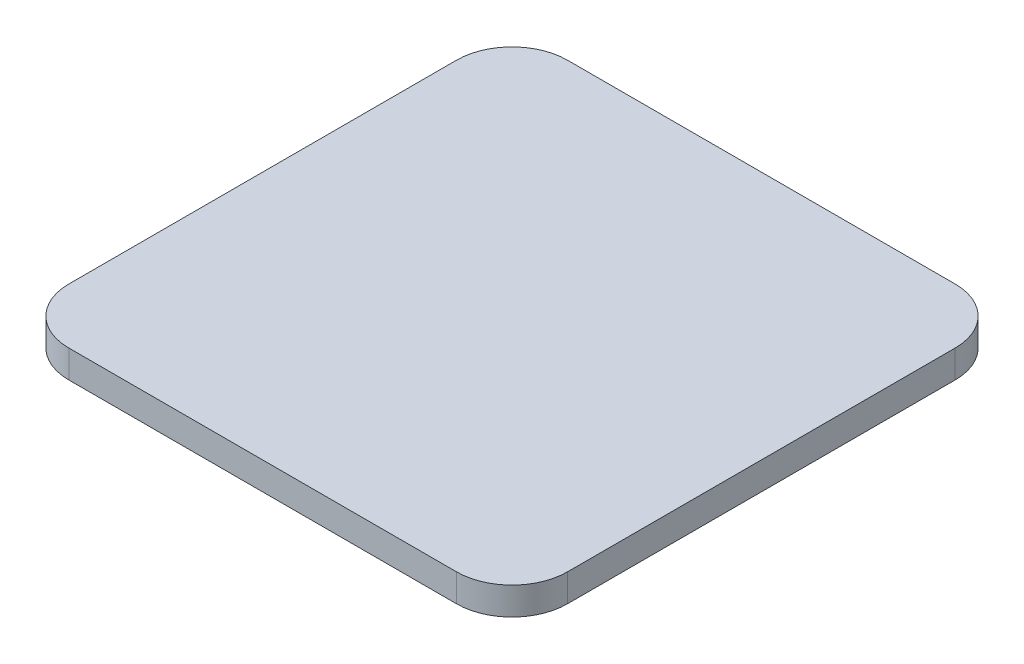
from build123d import *

# Parameters (mm, degrees)
SKETCH1_W           = 36
SKETCH1_H           = 36
BOSS_EXTRUDE1_DEPTH = 1
FILLET1_R           = 4


with BuildPart() as part:
    # Sketch1 → Boss-Extrude1 (new, symmetric)
    with BuildSketch(Plane(origin=(0, 0, 0), x_dir=(1, 0, 0), z_dir=(0, 1, 0))):
        Rectangle(SKETCH1_W, SKETCH1_H)
    extrude(amount=BOSS_EXTRUDE1_DEPTH, both=True)

    # Fillet1
    fillet1_edges = [part.edges().sort_by_distance(p)[0] for p in [
        (18, 0, 18),
        (-18, 0, 18),
        (-18, 0, -18),
        (18, 0, -18),
    ]]
    fillet(fillet1_edges, radius=FILLET1_R)


solid = part.part
